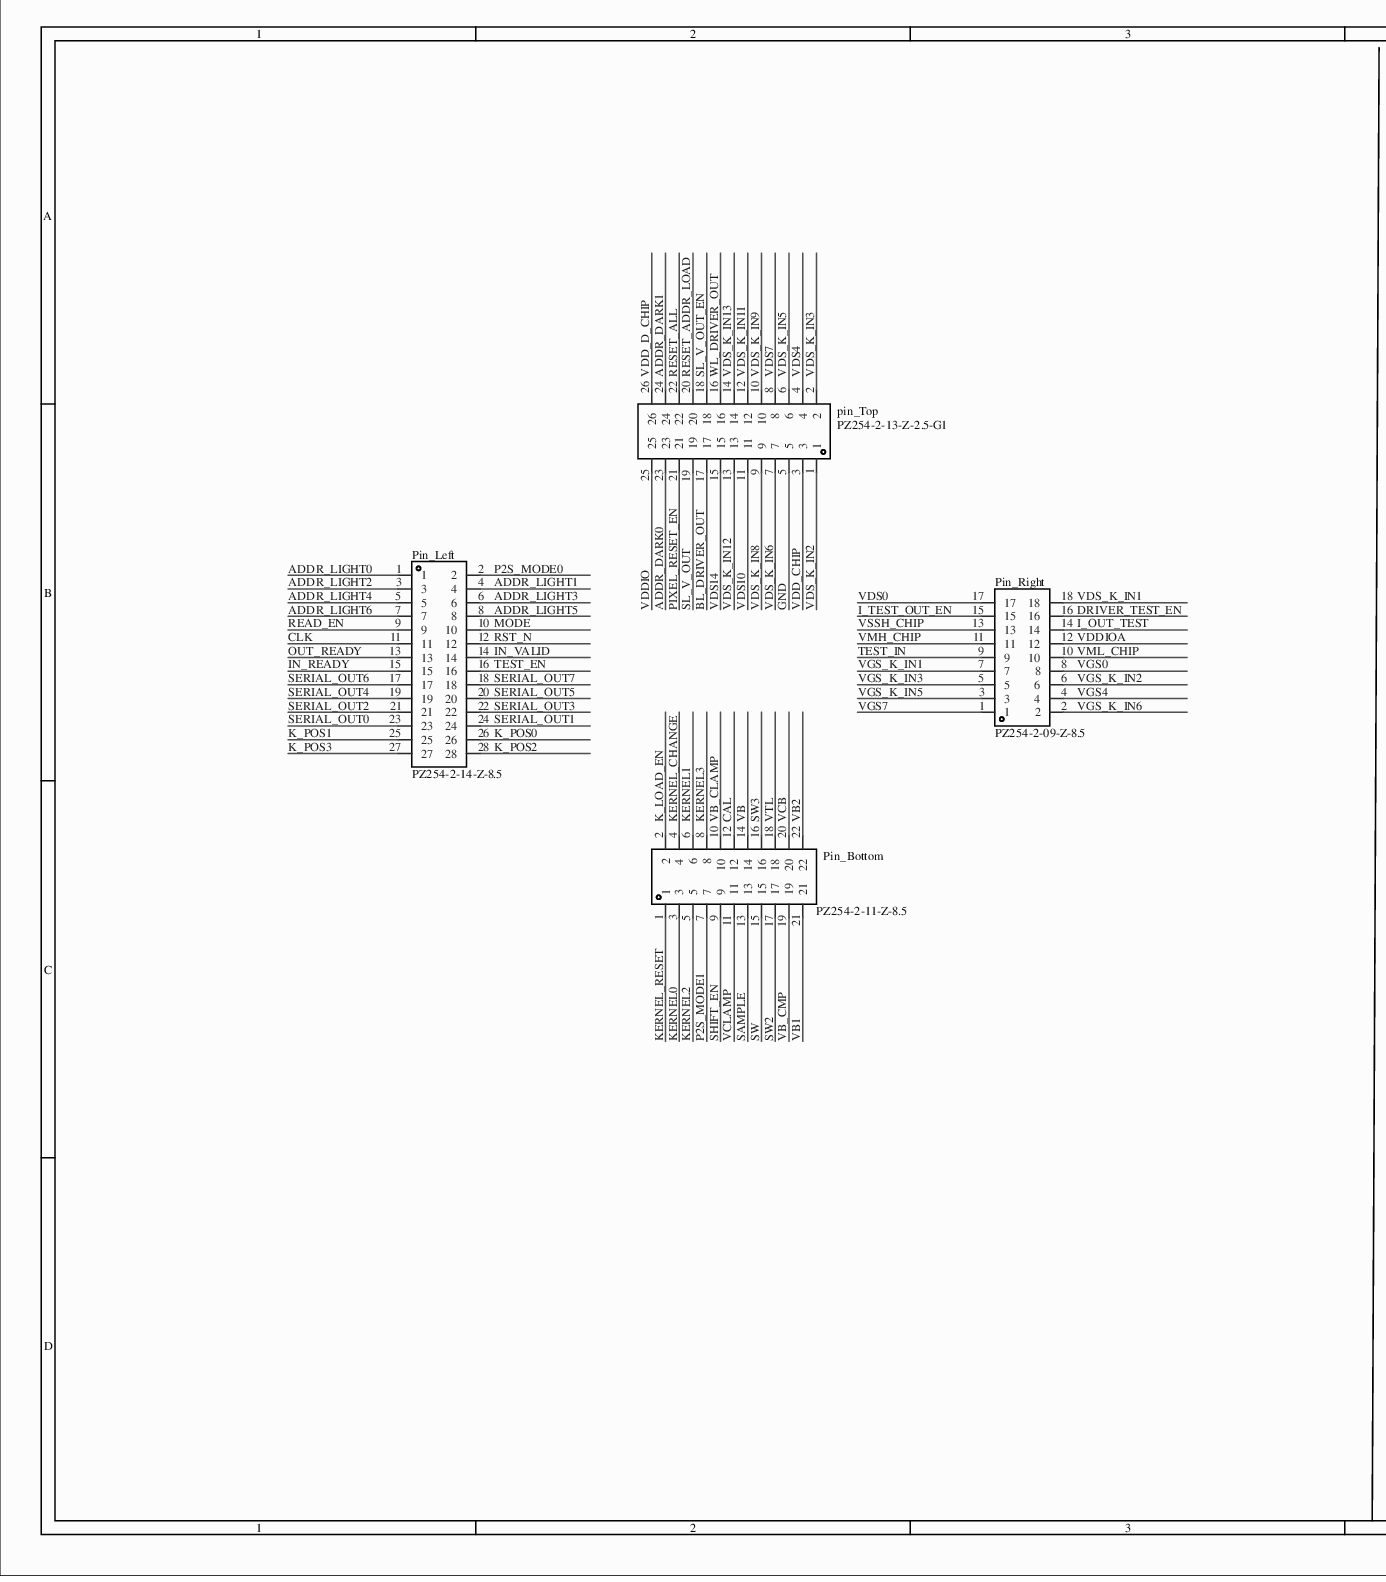
[diagram p0: MISC82784-2.schdoc, left]
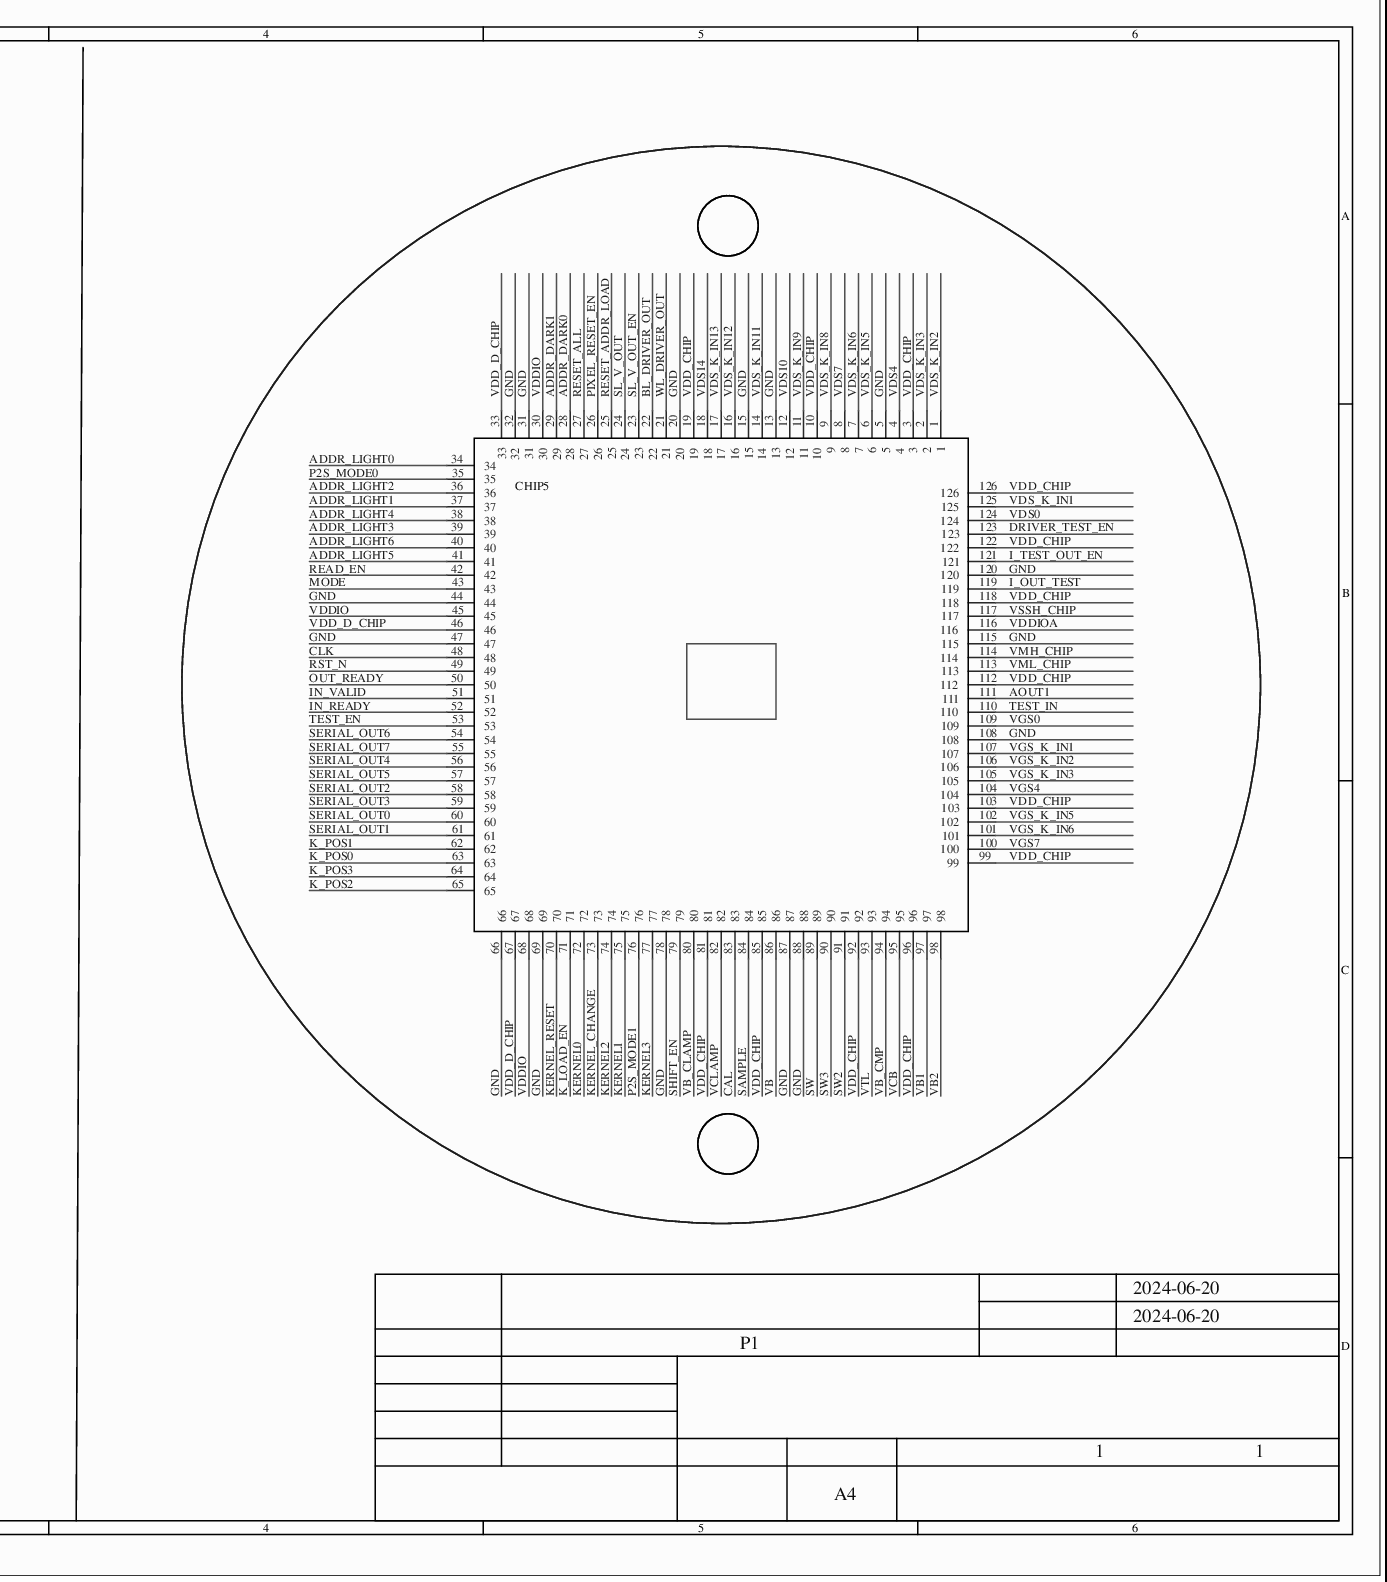
[diagram p1: MISC82784-2.schdoc, right]
# Altium project MISC82784-8.PrjPCB
1 sheet, 5 parts. Net scope: global (net labels, ports and power ports of the same name join across sheets).
Board file: MISC82784.pcbdoc

## Sheet MISC82784-2.schdoc
size 495 x 292 mm; Version: V1.0; @Project Name: MISC82784; @Page Count: 1; @Update Date: 2024-06-20; @Create Date: 2024-06-20; @Page No: 1

### Parts
CHIP5  chip5  [JSZ]  (value not drawn)
Pin_Bottom  PZ254-2-11-Z-8.5  [HDR2.54-LI-2x11P]
Pin_Left  PZ254-2-14-Z-8.5  [HDR2.54-LI-2x14P]
Pin_Right  PZ254-2-09-Z-8.5  [HDR2.54-LI-2x9P]
pin_Top  PZ254-2-13-Z-2.5-G1  [HDR2.54-LI-2x13P]

### Nets
ADDR_DARK0: CHIP5.28 pin_Top.23
ADDR_DARK1: CHIP5.29 pin_Top.24
ADDR_LIGHT0: CHIP5.34 Pin_Left.1
ADDR_LIGHT1: CHIP5.37 Pin_Left.4
ADDR_LIGHT2: CHIP5.36 Pin_Left.3
ADDR_LIGHT3: CHIP5.39 Pin_Left.6
ADDR_LIGHT4: CHIP5.38 Pin_Left.5
ADDR_LIGHT5: CHIP5.41 Pin_Left.8
ADDR_LIGHT6: CHIP5.40 Pin_Left.7
AOUT1: CHIP5.111
BL_DRIVER_OUT: CHIP5.22 pin_Top.17
CAL: CHIP5.83 Pin_Bottom.12
CLK: CHIP5.48 Pin_Left.11
DRIVER_TEST_EN: CHIP5.123 Pin_Right.16
GND: CHIP5.5 CHIP5.13 CHIP5.15 CHIP5.20 CHIP5.31 CHIP5.32 CHIP5.44 CHIP5.47 CHIP5.66 CHIP5.69 CHIP5.78 CHIP5.87 CHIP5.88 CHIP5.108 CHIP5.115 CHIP5.120 pin_Top.5
I_OUT_TEST: CHIP5.119 Pin_Right.14
I_TEST_OUT_EN: CHIP5.121 Pin_Right.15
IN_READY: CHIP5.52 Pin_Left.15
IN_VALID: CHIP5.51 Pin_Left.14
K_LOAD_EN: CHIP5.71 Pin_Bottom.2
K_POS0: CHIP5.63 Pin_Left.26
K_POS1: CHIP5.62 Pin_Left.25
K_POS2: CHIP5.65 Pin_Left.28
K_POS3: CHIP5.64 Pin_Left.27
KERNEL0: CHIP5.72 Pin_Bottom.3
KERNEL1: CHIP5.75 Pin_Bottom.6
KERNEL2: CHIP5.74 Pin_Bottom.5
KERNEL3: CHIP5.77 Pin_Bottom.8
KERNEL_CHANGE: CHIP5.73 Pin_Bottom.4
KERNEL_RESET: CHIP5.70 Pin_Bottom.1
MODE: CHIP5.43 Pin_Left.10
OUT_READY: CHIP5.50 Pin_Left.13
P2S_MODE0: CHIP5.35 Pin_Left.2
P2S_MODE1: CHIP5.76 Pin_Bottom.7
PIXEL_RESET_EN: CHIP5.26 pin_Top.21
READ_EN: CHIP5.42 Pin_Left.9
RESET_ADDR_LOAD: CHIP5.25 pin_Top.20
RESET_ALL: CHIP5.27 pin_Top.22
RST_N: CHIP5.49 Pin_Left.12
SAMPLE: CHIP5.84 Pin_Bottom.13
SERIAL_OUT0: CHIP5.60 Pin_Left.23
SERIAL_OUT1: CHIP5.61 Pin_Left.24
SERIAL_OUT2: CHIP5.58 Pin_Left.21
SERIAL_OUT3: CHIP5.59 Pin_Left.22
SERIAL_OUT4: CHIP5.56 Pin_Left.19
SERIAL_OUT5: CHIP5.57 Pin_Left.20
SERIAL_OUT6: CHIP5.54 Pin_Left.17
SERIAL_OUT7: CHIP5.55 Pin_Left.18
SHIFT_EN: CHIP5.79 Pin_Bottom.9
SL_V_OUT: CHIP5.24 pin_Top.19
SL_V_OUT_EN: CHIP5.23 pin_Top.18
SW: CHIP5.89 Pin_Bottom.15
SW2: CHIP5.91 Pin_Bottom.17
SW3: CHIP5.90 Pin_Bottom.16
TEST_EN: CHIP5.53 Pin_Left.16
TEST_IN: CHIP5.110 Pin_Right.9
VB: CHIP5.86 Pin_Bottom.14
VB1: CHIP5.97 Pin_Bottom.21
VB2: CHIP5.98 Pin_Bottom.22
VB_CLAMP: CHIP5.80 Pin_Bottom.10
VB_CMP: CHIP5.94 Pin_Bottom.19
VCB: CHIP5.95 Pin_Bottom.20
VCLAMP: CHIP5.82 Pin_Bottom.11
VDD_CHIP: CHIP5.3 CHIP5.10 CHIP5.19 CHIP5.81 CHIP5.85 CHIP5.92 CHIP5.96 CHIP5.99 CHIP5.103 CHIP5.112 CHIP5.118 CHIP5.122 CHIP5.126 pin_Top.3
VDD_D_CHIP: CHIP5.33 CHIP5.46 CHIP5.67 pin_Top.26
VDDIO: CHIP5.30 CHIP5.45 CHIP5.68 pin_Top.25
VDDIOA: CHIP5.116 Pin_Right.12
VDS0: CHIP5.124 Pin_Right.17
VDS4: CHIP5.4 pin_Top.4
VDS7: CHIP5.8 pin_Top.8
VDS10: CHIP5.12 pin_Top.11
VDS14: CHIP5.18 pin_Top.15
VDS_K_IN1: CHIP5.125 Pin_Right.18
VDS_K_IN2: CHIP5.1 pin_Top.1
VDS_K_IN3: CHIP5.2 pin_Top.2
VDS_K_IN5: CHIP5.6 pin_Top.6
VDS_K_IN6: CHIP5.7 pin_Top.7
VDS_K_IN8: CHIP5.9 pin_Top.9
VDS_K_IN9: CHIP5.11 pin_Top.10
VDS_K_IN11: CHIP5.14 pin_Top.12
VDS_K_IN12: CHIP5.16 pin_Top.13
VDS_K_IN13: CHIP5.17 pin_Top.14
VGS0: CHIP5.109 Pin_Right.8
VGS4: CHIP5.104 Pin_Right.4
VGS7: CHIP5.100 Pin_Right.1
VGS_K_IN1: CHIP5.107 Pin_Right.7
VGS_K_IN2: CHIP5.106 Pin_Right.6
VGS_K_IN3: CHIP5.105 Pin_Right.5
VGS_K_IN5: CHIP5.102 Pin_Right.3
VGS_K_IN6: CHIP5.101 Pin_Right.2
VMH_CHIP: CHIP5.114 Pin_Right.11
VML_CHIP: CHIP5.113 Pin_Right.10
VSSH_CHIP: CHIP5.117 Pin_Right.13
VTL: CHIP5.93 Pin_Bottom.18
WL_DRIVER_OUT: CHIP5.21 pin_Top.16

### Notes on the sheet
- 1
- 2
- 3
- 4
- 5
- 6
- A
- B
- C
- 2024-06-20
- D
- P1
- A4

### Library data of the parts
CHIP5 = chip5: Add into BOM: yes; Symbol: chip5; Device: chip5; Convert to PCB: yes
Pin_Bottom = PZ254-2-11-Z-8.5: Add into BOM: yes; Pin Structure: 2x11P; Pitch: 2.54mm; Current Rating (Max): 3A; Name: PZ254-2-11-Z-8.5; Symbol: PZ254-2-11-Z-8.5; Device: PZ254-2-11-Z-8.5; Supplier Part: C2894972; Manufacturer Part: PZ254-2-11-Z-8.5; Datasheet: example.com/20230609/5BA09C8BEB9B31376F8BF6032FF67CAC.pdf; Supplier: LCSC; Convert to PCB: yes; Row Spacing: 2.54mm; Number of Pins: 22P; Voltage Rating (Max): -; Length of Mating Pin: 6mm; Insulation Height: 2.5mm; Length of End Connection Pin: 3mm
Pin_Left = PZ254-2-14-Z-8.5: Add into BOM: yes; Pin Structure: 2x14P; Pitch: 2.54mm; Current Rating (Max): 3A; Name: PZ254-2-14-Z-8.5; Symbol: PZ254-2-14-Z-8.5; Device: PZ254-2-14-Z-8.5; Supplier Part: C2894975; Manufacturer Part: PZ254-2-14-Z-8.5; Datasheet: example.com/20230609/5BA09C8BEB9B31376F8BF6032FF67CAC.pdf; Supplier: LCSC; Convert to PCB: yes; Row Spacing: 2.54mm; Number of Pins: 28P; Voltage Rating (Max): -; Length of Mating Pin: 6mm; Insulation Height: 2.5mm; Length of End Connection Pin: 3mm
Pin_Right = PZ254-2-09-Z-8.5: Add into BOM: yes; Pin Structure: 2x9P; Pitch: 2.54mm; Current Rating (Max): 3A; Name: PZ254-2-09-Z-8.5; Symbol: PZ254-2-09-Z-8.5; Device: PZ254-2-09-Z-8.5; Supplier Part: C2894970; Manufacturer Part: PZ254-2-09-Z-8.5; Datasheet: example.com/20230609/5BA09C8BEB9B31376F8BF6032FF67CAC.pdf; Supplier: LCSC; Convert to PCB: yes; Row Spacing: 2.54mm; Number of Pins: 18P; Voltage Rating (Max): -; Length of Mating Pin: 6mm; Insulation Height: 2.5mm; Length of End Connection Pin: 3mm
pin_Top = PZ254-2-13-Z-2.5-G1: Add into BOM: yes; Pin Structure: 2x13P; Pitch: 2.54mm; Current Rating (Max): 3A; Name: PZ254-2-13-Z-2.5-G1; Symbol: PZ254-2-13-Z-2.5-G1; Device: PZ254-2-13-Z-2.5-G1; Supplier: LCSC; Supplier Part: C18198008; Manufacturer Part: PZ254-2-13-Z-2.5-G1; Datasheet: example.com/20230921/D8C53D635FAFF8233B09D1367D616037.pdf; Convert to PCB: yes; Row Spacing: 2.54mm; Number of Pins: 26P; Length of Mating Pin: 6mm; Insulation Height: 2.5mm; Length of End Connection Pin: 3mm